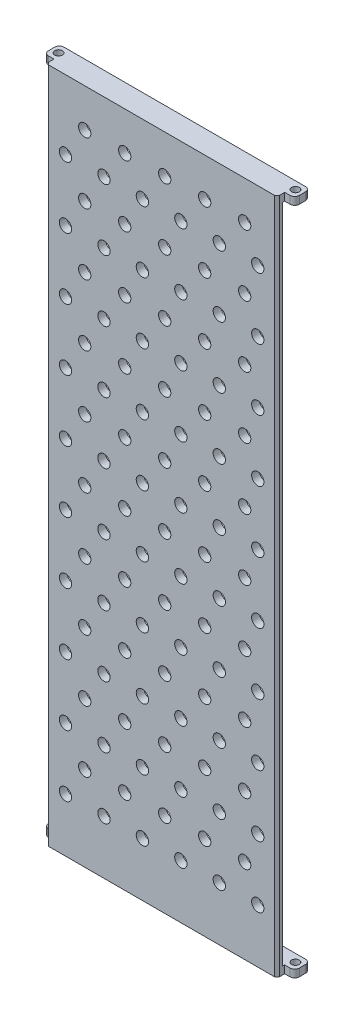
from build123d import *

# Parameters (mm, degrees)
SKETCH1_W               = 150
SKETCH1_H               = 430
BOSS_EXTRUDE1_DEPTH     = 5
CUT_EXTRUDE1_REACH      = 457.439
SKETCH2_R               = 4
LPATTERN1_COUNT         = 10
LPATTERN1_PITCH         = 40
SKETCH3_W               = 163
SKETCH3_H               = 15
BOSS_EXTRUDE2_DEPTH     = 5
SKETCH4_W               = 163
SKETCH4_H               = 15
BOSS_EXTRUDE3_DEPTH     = 5
CUT_EXTRUDE2_DEPTH      = 468.110532958
CUT_EXTRUDE2_DEPTH_BACK = 468.110532958
SKETCH6_R               = 2.5
SKETCH6_W               = 6.5
SKETCH6_H               = 5
FILLET1_R               = 3
CHAMFER1_SIZE           = 1.5


with BuildPart() as part:
    # Sketch1 → Boss-Extrude1 (new body)
    with BuildSketch(Plane.XY):
        with Locations((75, 215)):
            Rectangle(SKETCH1_W, SKETCH1_H)
    extrude(amount=BOSS_EXTRUDE1_DEPTH)

    # Sketch2 → Cut-Extrude1 (cut, up to next)
    with BuildSketch(Plane.XY.offset(5), mode=Mode.PRIVATE) as cut_extrude1_sk1:
        with Locations((25, 410)):
            Circle(SKETCH2_R)
    cut_extrude1_tool1 = extrude(cut_extrude1_sk1.sketch, amount=-CUT_EXTRUDE1_REACH, mode=Mode.PRIVATE) & part.part
    # Sketch2 → Cut-Extrude1 (cut, up to next)
    with BuildSketch(Plane.XY.offset(5), mode=Mode.PRIVATE) as cut_extrude1_sk2:
        with Locations((51, 410)):
            Circle(SKETCH2_R)
    cut_extrude1_tool2 = extrude(cut_extrude1_sk2.sketch, amount=-CUT_EXTRUDE1_REACH, mode=Mode.PRIVATE) & part.part
    # Sketch2 → Cut-Extrude1 (cut, up to next)
    with BuildSketch(Plane.XY.offset(5), mode=Mode.PRIVATE) as cut_extrude1_sk3:
        with Locations((77, 410)):
            Circle(SKETCH2_R)
    cut_extrude1_tool3 = extrude(cut_extrude1_sk3.sketch, amount=-CUT_EXTRUDE1_REACH, mode=Mode.PRIVATE) & part.part
    # Sketch2 → Cut-Extrude1 (cut, up to next)
    with BuildSketch(Plane.XY.offset(5), mode=Mode.PRIVATE) as cut_extrude1_sk4:
        with Locations((103, 410)):
            Circle(SKETCH2_R)
    cut_extrude1_tool4 = extrude(cut_extrude1_sk4.sketch, amount=-CUT_EXTRUDE1_REACH, mode=Mode.PRIVATE) & part.part
    # Sketch2 → Cut-Extrude1 (cut, up to next)
    with BuildSketch(Plane.XY.offset(5), mode=Mode.PRIVATE) as cut_extrude1_sk5:
        with Locations((129, 410)):
            Circle(SKETCH2_R)
    cut_extrude1_tool5 = extrude(cut_extrude1_sk5.sketch, amount=-CUT_EXTRUDE1_REACH, mode=Mode.PRIVATE) & part.part
    # Sketch2 → Cut-Extrude1 (cut, up to next)
    with BuildSketch(Plane.XY.offset(5), mode=Mode.PRIVATE) as cut_extrude1_sk6:
        with Locations((12.5, 390)):
            Circle(SKETCH2_R)
    cut_extrude1_tool6 = extrude(cut_extrude1_sk6.sketch, amount=-CUT_EXTRUDE1_REACH, mode=Mode.PRIVATE) & part.part
    # Sketch2 → Cut-Extrude1 (cut, up to next)
    with BuildSketch(Plane.XY.offset(5), mode=Mode.PRIVATE) as cut_extrude1_sk7:
        with Locations((37.5, 390)):
            Circle(SKETCH2_R)
    cut_extrude1_tool7 = extrude(cut_extrude1_sk7.sketch, amount=-CUT_EXTRUDE1_REACH, mode=Mode.PRIVATE) & part.part
    # Sketch2 → Cut-Extrude1 (cut, up to next)
    with BuildSketch(Plane.XY.offset(5), mode=Mode.PRIVATE) as cut_extrude1_sk8:
        with Locations((62.5, 390)):
            Circle(SKETCH2_R)
    cut_extrude1_tool8 = extrude(cut_extrude1_sk8.sketch, amount=-CUT_EXTRUDE1_REACH, mode=Mode.PRIVATE) & part.part
    # Sketch2 → Cut-Extrude1 (cut, up to next)
    with BuildSketch(Plane.XY.offset(5), mode=Mode.PRIVATE) as cut_extrude1_sk9:
        with Locations((87.5, 390)):
            Circle(SKETCH2_R)
    cut_extrude1_tool9 = extrude(cut_extrude1_sk9.sketch, amount=-CUT_EXTRUDE1_REACH, mode=Mode.PRIVATE) & part.part
    # Sketch2 → Cut-Extrude1 (cut, up to next)
    with BuildSketch(Plane.XY.offset(5), mode=Mode.PRIVATE) as cut_extrude1_sk10:
        with Locations((112.5, 390)):
            Circle(SKETCH2_R)
    cut_extrude1_tool10 = extrude(cut_extrude1_sk10.sketch, amount=-CUT_EXTRUDE1_REACH, mode=Mode.PRIVATE) & part.part
    # Sketch2 → Cut-Extrude1 (cut, up to next)
    with BuildSketch(Plane.XY.offset(5), mode=Mode.PRIVATE) as cut_extrude1_sk11:
        with Locations((137.5, 390)):
            Circle(SKETCH2_R)
    cut_extrude1_tool11 = extrude(cut_extrude1_sk11.sketch, amount=-CUT_EXTRUDE1_REACH, mode=Mode.PRIVATE) & part.part
    cut_extrude1_1 = cut_extrude1_tool1.solids().sort_by_distance((25, 410, 5))[0]
    add(cut_extrude1_1, mode=Mode.SUBTRACT)
    cut_extrude1_2 = cut_extrude1_tool2.solids().sort_by_distance((51, 410, 5))[0]
    add(cut_extrude1_2, mode=Mode.SUBTRACT)
    cut_extrude1_3 = cut_extrude1_tool3.solids().sort_by_distance((77, 410, 5))[0]
    add(cut_extrude1_3, mode=Mode.SUBTRACT)
    cut_extrude1_4 = cut_extrude1_tool4.solids().sort_by_distance((103, 410, 5))[0]
    add(cut_extrude1_4, mode=Mode.SUBTRACT)
    cut_extrude1_5 = cut_extrude1_tool5.solids().sort_by_distance((129, 410, 5))[0]
    add(cut_extrude1_5, mode=Mode.SUBTRACT)
    cut_extrude1_6 = cut_extrude1_tool6.solids().sort_by_distance((12.5, 390, 5))[0]
    add(cut_extrude1_6, mode=Mode.SUBTRACT)
    cut_extrude1_7 = cut_extrude1_tool7.solids().sort_by_distance((37.5, 390, 5))[0]
    add(cut_extrude1_7, mode=Mode.SUBTRACT)
    cut_extrude1_8 = cut_extrude1_tool8.solids().sort_by_distance((62.5, 390, 5))[0]
    add(cut_extrude1_8, mode=Mode.SUBTRACT)
    cut_extrude1_9 = cut_extrude1_tool9.solids().sort_by_distance((87.5, 390, 5))[0]
    add(cut_extrude1_9, mode=Mode.SUBTRACT)
    cut_extrude1_10 = cut_extrude1_tool10.solids().sort_by_distance((112.5, 390, 5))[0]
    add(cut_extrude1_10, mode=Mode.SUBTRACT)
    cut_extrude1_11 = cut_extrude1_tool11.solids().sort_by_distance((137.5, 390, 5))[0]
    add(cut_extrude1_11, mode=Mode.SUBTRACT)
    cut_extrude1 = cut_extrude1_1 + cut_extrude1_2 + cut_extrude1_3 + cut_extrude1_4 + cut_extrude1_5 + cut_extrude1_6 + cut_extrude1_7 + cut_extrude1_8 + cut_extrude1_9 + cut_extrude1_10 + cut_extrude1_11  # Cut-Extrude1 as one shape, for the pattern or mirror that repeats it

    # LPattern1: Cut-Extrude1 ×10
    with Locations(*[(0, -i * LPATTERN1_PITCH, 0) for i in range(1, LPATTERN1_COUNT)]):
        add(cut_extrude1, mode=Mode.SUBTRACT)

    # Sketch3 → Boss-Extrude2 (add)
    with BuildSketch(Plane(origin=(0, 0, 0), x_dir=(-1, 0, 0), z_dir=(0, -1, 0))):
        with Locations((-75, 2.5)):
            Rectangle(SKETCH3_W, SKETCH3_H)
    extrude(amount=BOSS_EXTRUDE2_DEPTH)

    # Sketch4 → Boss-Extrude3 (add)
    with BuildSketch(Plane(origin=(0, 430, 0), x_dir=(1, 0, 0), z_dir=(0, 1, 0))):
        with Locations((75, 2.5)):
            Rectangle(SKETCH4_W, SKETCH4_H)
    extrude(amount=BOSS_EXTRUDE3_DEPTH)

    # Sketch6 → Cut-Extrude2 (cut, two sides: drawn at the far end of the back side and taken through both)
    with BuildSketch(Plane(origin=(0, 435, 0), x_dir=(1, 0, 0), z_dir=(0, 1, 0)).offset(-CUT_EXTRUDE2_DEPTH_BACK)):
        with Locations(Location((-2, 5, 0), (0, 0, 270))):
            Circle(SKETCH6_R)
        with Locations(Location((152, 5, 0), (0, 0, 270))):
            Circle(SKETCH6_R)
        with Locations((153.25, -2.5)):
            Rectangle(SKETCH6_W, SKETCH6_H)
        with Locations((-3.25, -2.5)):
            Rectangle(SKETCH6_W, SKETCH6_H)
    extrude(amount=CUT_EXTRUDE2_DEPTH + CUT_EXTRUDE2_DEPTH_BACK, mode=Mode.SUBTRACT)

    # Fillet1
    fillet1_edges = [part.edges().sort_by_distance(p)[0] for p in [
        (-6.5, -2.5, -10),
        (156.5, -2.5, -10),
        (-6.5, 432.5, -10),
        (156.5, 432.5, -10),
        (-6.5, 432.5, 0),
        (-6.5, -2.5, 0),
        (156.5, 432.5, 0),
        (156.5, -2.5, 0),
    ]]
    fillet(fillet1_edges, radius=FILLET1_R)

    # Chamfer1
    chamfer1_edges = [part.edges().sort_by_distance(p)[0] for p in [
        (150, 215, 5),
        (0, 215, 5),
        (150, 215, 0),
        (0, 215, 0),
    ]]
    chamfer(chamfer1_edges, length=CHAMFER1_SIZE)


solid = part.part
